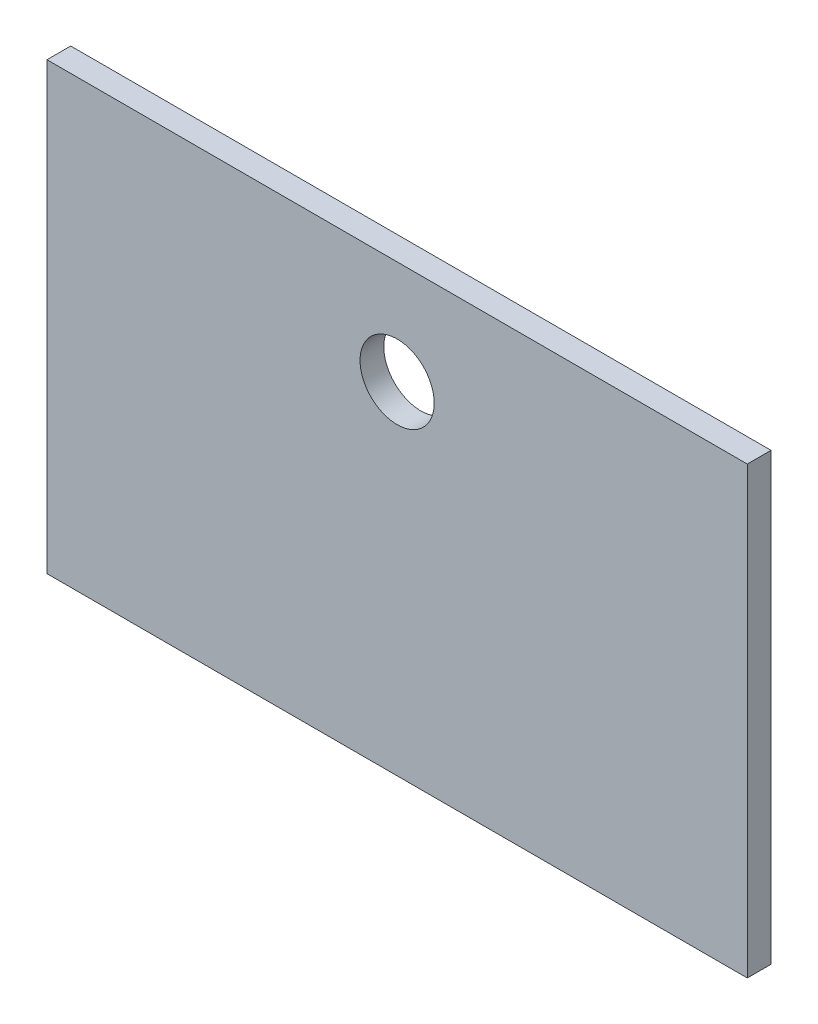
from build123d import *

# Parameters (mm, degrees)
SKETCH1_W                  = 236
SKETCH1_H                  = 150
BOSS_EXTRUDE1_DEPTH        = 4
F_25_0_25_DIAMETER_HOLE1_D = 25


with BuildPart() as part:
    # Sketch1 → Boss-Extrude1 (new, symmetric)
    with BuildSketch(Plane.XY):
        Rectangle(SKETCH1_W, SKETCH1_H)
    extrude(amount=BOSS_EXTRUDE1_DEPTH, both=True)

    # Ø25.0 (25) Diameter Hole1 (through all)
    with Locations(Plane.XY.offset(4)):
        with Locations((0, 40)):
            Hole(F_25_0_25_DIAMETER_HOLE1_D / 2)


solid = part.part
